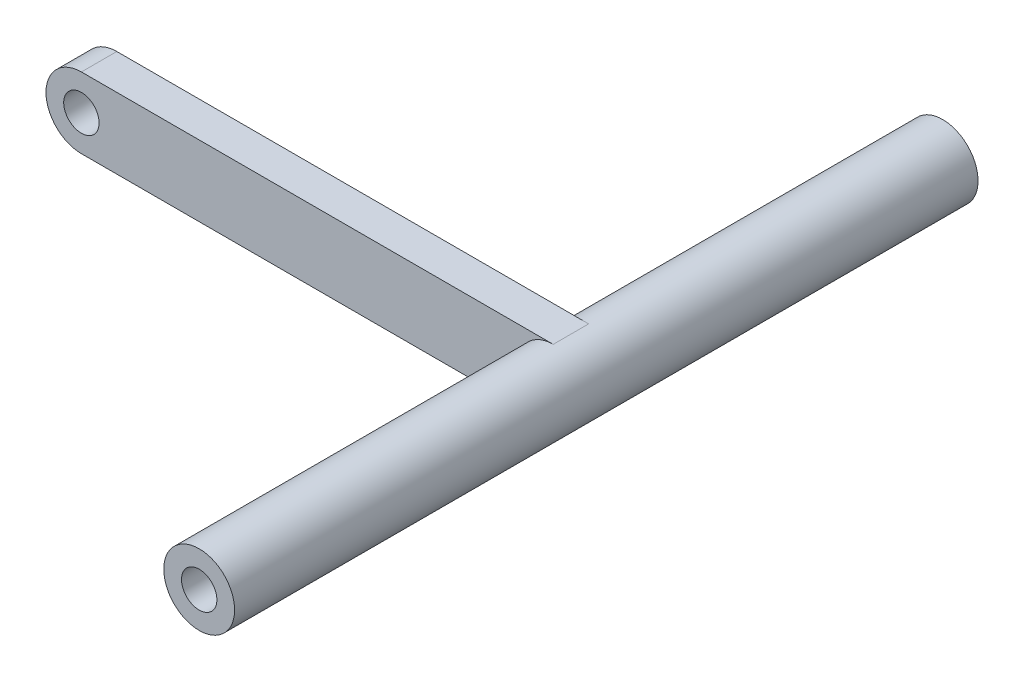
SolidWorks part; units mm, degrees
material "1060 合金"
ref_plane "前视基准面" through (0, 0, 0) normal (0, 0, 1) x (1, 0, 0)
ref_plane "上视基准面" through (0, 0, 0) normal (0, 1, 0) x (1, 0, 0)
ref_plane "右视基准面" through (0, 0, 0) normal (1, 0, 0) x (0, 0, -1)
other "Configuration Table"
sketch "草图1" plane through (0, 0, 0) normal (0, 0, 1) x (1, 0, 0)
  line L0 (-66.635, 0) -> (66.635, 0) construction
  line L1 (-66.635, 10) -> (66.635, 10)
  line L2 (-66.635, -10) -> (66.635, -10)
  arc A0 (-66.635, 10) -> (-66.635, -10) centre (-66.635, 0) ccw
  arc A1 (66.635, -10) -> (66.635, 10) centre (66.635, 0) ccw
  circle A4 centre (-66.635, 0) radius 5
  circle A5 centre (66.635, 0) radius 4.3761
  point P2 (0, 0)
  dimension "D3" = 10
  dimension "D1" = 20
  dimension "D2" = 133.27
extrude "凸台-拉伸1" add sketch "草图1" along normal blind 10
sketch "草图2" plane through (0, 0, 10) normal (0, 0, 1) x (1, 0, 0)
  circle A0 centre (66.635, 0) radius 10
  dimension "D1" = 20
extrude "凸台-拉伸2" add sketch "草图2" along normal blind 100
sketch "草图3" plane through (0, 0, 0) normal (0, 0, -1) x (-1, 0, 0)
  circle A0 centre (-66.635, 0) radius 10
  dimension "D1" = 20
extrude "凸台-拉伸3" add sketch "草图3" along normal blind 100
sketch "草图4" plane through (0, 0, -100) normal (0, 0, -1) x (-1, 0, 0)
  circle A0 centre (-66.635, 0) radius 5
  dimension "D1" = 10
extrude "切除-拉伸1" cut sketch "草图4" against normal through all both and the other way through all
